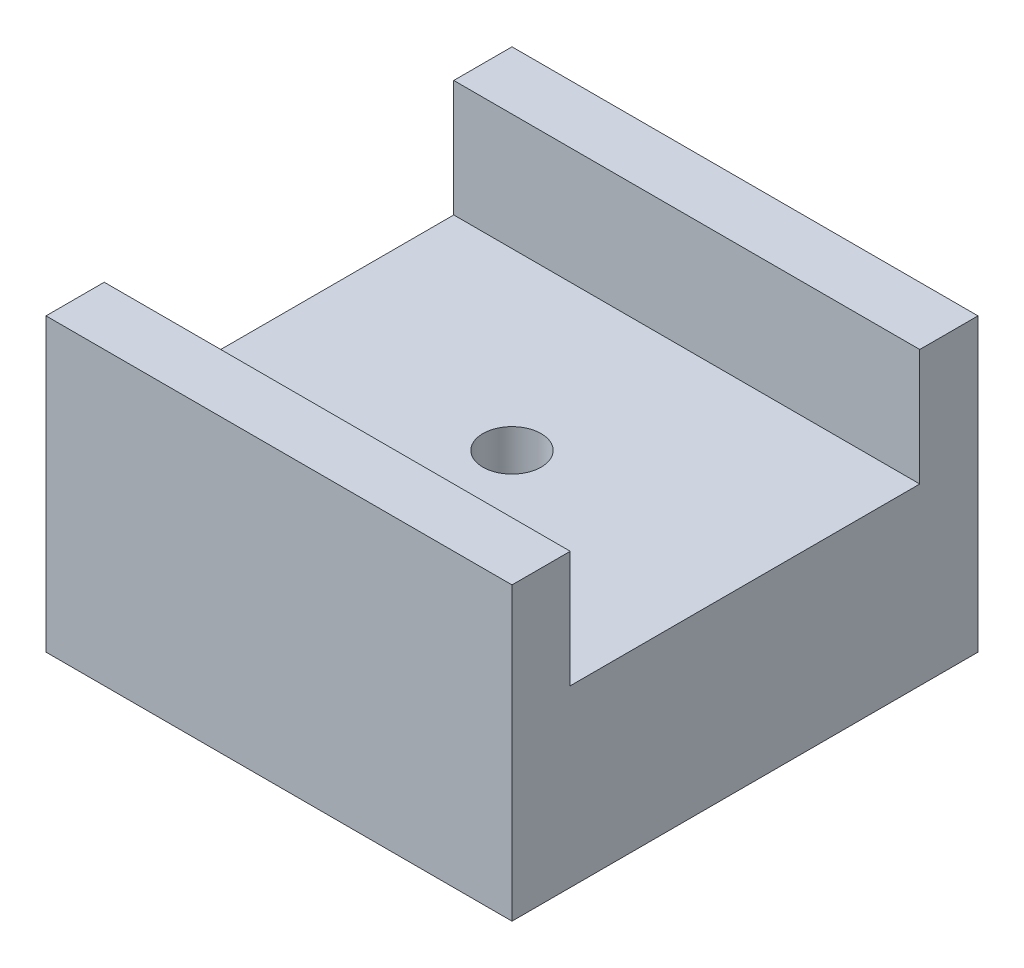
from build123d import *

# Parameters (mm, degrees)
SKETCH1_W           = 40
SKETCH1_H           = 40
BOSS_EXTRUDE1_DEPTH = 25
SKETCH2_W           = 40
SKETCH2_H           = 30
CUT_EXTRUDE1_DEPTH  = 10
M6_TAPPED_HOLE1_D   = 5


with BuildPart() as part:
    # Sketch1 → Boss-Extrude1 (new body)
    with BuildSketch(Plane(origin=(0, 0, 0), x_dir=(1, 0, 0), z_dir=(0, 1, 0))):
        Rectangle(SKETCH1_W, SKETCH1_H)
    extrude(amount=BOSS_EXTRUDE1_DEPTH)

    # Sketch2 → Cut-Extrude1 (cut)
    with BuildSketch(Plane(origin=(0, 25, 0), x_dir=(1, 0, 0), z_dir=(0, 1, 0))):
        Rectangle(SKETCH2_W, SKETCH2_H)
    extrude(amount=-CUT_EXTRUDE1_DEPTH, mode=Mode.SUBTRACT)

    # M6 Tapped Hole1 (through all)
    with Locations(Plane(origin=(0, 0, 0), x_dir=(-1, 0, 0), z_dir=(0, -1, 0))):
        with Locations((0, 0)):
            Hole(M6_TAPPED_HOLE1_D / 2)


solid = part.part
